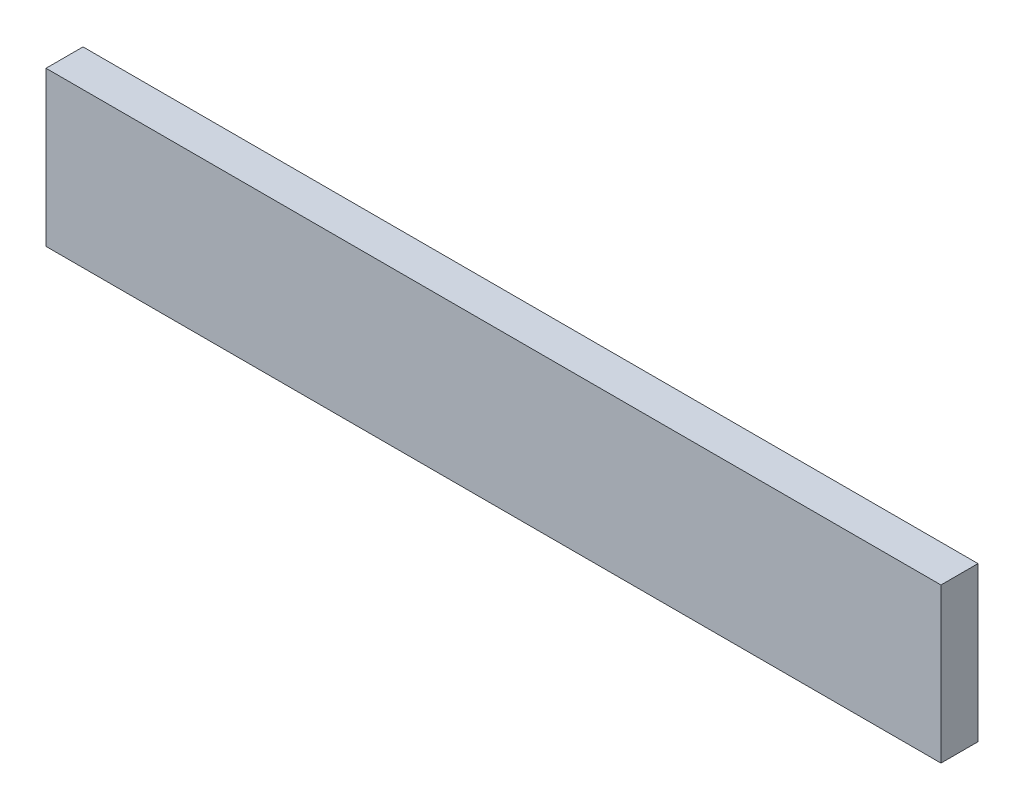
SolidWorks part; units mm, degrees
material "Q235"
ref_plane "Front Plane" through (0, 0, 0) normal (0, 0, 1) x (1, 0, 0)
ref_plane "Top Plane" through (0, 0, 0) normal (0, 1, 0) x (1, 0, 0)
ref_plane "Right Plane" through (0, 0, 0) normal (1, 0, 0) x (0, 0, -1)
sketch "Sketch1" plane through (0, 0, 0) normal (0, 0, 1) x (1, 0, 0)
  line L1 (0, 0) -> (290, 0)
  line L2 (0, 0) -> (0, 50)
  line L3 (0, 50) -> (290, 50)
  line L4 (290, 0) -> (290, 50)
  dimension "D1" = 290
  dimension "D2" = 50
extrude "Boss-Extrude1" add sketch "Sketch1" along normal blind 12
